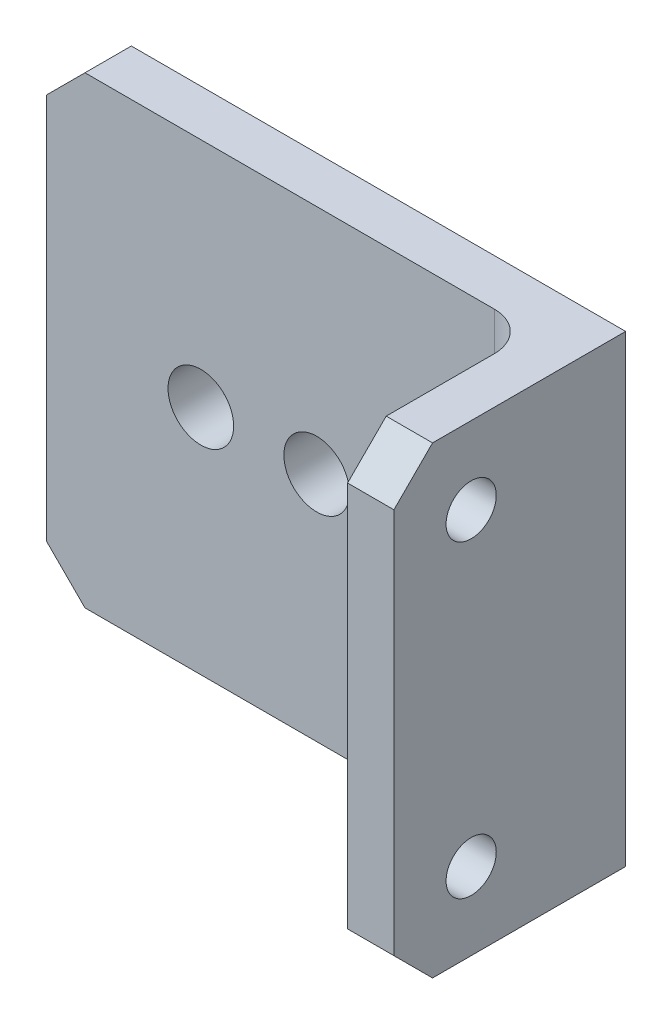
from build123d import *

# Parameters (mm, degrees)
SKETCH1_W           = 69
SKETCH1_H           = 60
BOSS_EXTRUDE1_DEPTH = 3
SKETCH2_W           = 6
SKETCH2_H           = 60
BOSS_EXTRUDE2_DEPTH = 24
CHAMFER1_SIZE       = 5
SKETCH3_R           = 4.25
CUT_EXTRUDE1_DEPTH  = 52.635743434
FILLET1_R           = 5
SKETCH4_R           = 3.25
CUT_EXTRUDE2_DEPTH  = 75.81978348


with BuildPart() as part:
    # Sketch1 → Boss-Extrude1 (new, symmetric)
    with BuildSketch(Plane.XY):
        Rectangle(SKETCH1_W, SKETCH1_H)
    extrude(amount=BOSS_EXTRUDE1_DEPTH, both=True)

    # Sketch2 → Boss-Extrude2 (add)
    with BuildSketch(Plane.XY.offset(3)):
        with Locations((31.5, 0)):
            Rectangle(SKETCH2_W, SKETCH2_H)
    extrude(amount=BOSS_EXTRUDE2_DEPTH)

    # Chamfer1
    chamfer1_edges = [part.edges().sort_by_distance(p)[0] for p in [
        (31.5, 30, 27),
        (31.5, -30, 27),
        (-34.5, 30, 0),
        (-34.5, -30, 0),
    ]]
    chamfer(chamfer1_edges, length=CHAMFER1_SIZE)

    # Sketch3 → Cut-Extrude1 (cut, through all)
    with BuildSketch(Plane.XY.offset(3)):
        with Locations((-14.5, 0)):
            Circle(SKETCH3_R)
        with Locations((0.5, 0)):
            Circle(SKETCH3_R)
    extrude(amount=-CUT_EXTRUDE1_DEPTH, mode=Mode.SUBTRACT)

    # Fillet1
    fillet1_edges = [part.edges().sort_by_distance(p)[0] for p in [
        (28.5, 0, 3),
    ]]
    fillet(fillet1_edges, radius=FILLET1_R)

    # Sketch4 → Cut-Extrude2 (cut, through all)
    with BuildSketch(Plane.ZY.offset(-28.5)):
        with Locations(Location((17, 20, 0), (0, 0, 270))):
            Circle(SKETCH4_R)
        with Locations(Location((17, -20, 0), (0, 0, 270))):
            Circle(SKETCH4_R)
    extrude(amount=-CUT_EXTRUDE2_DEPTH, mode=Mode.SUBTRACT)


solid = part.part
